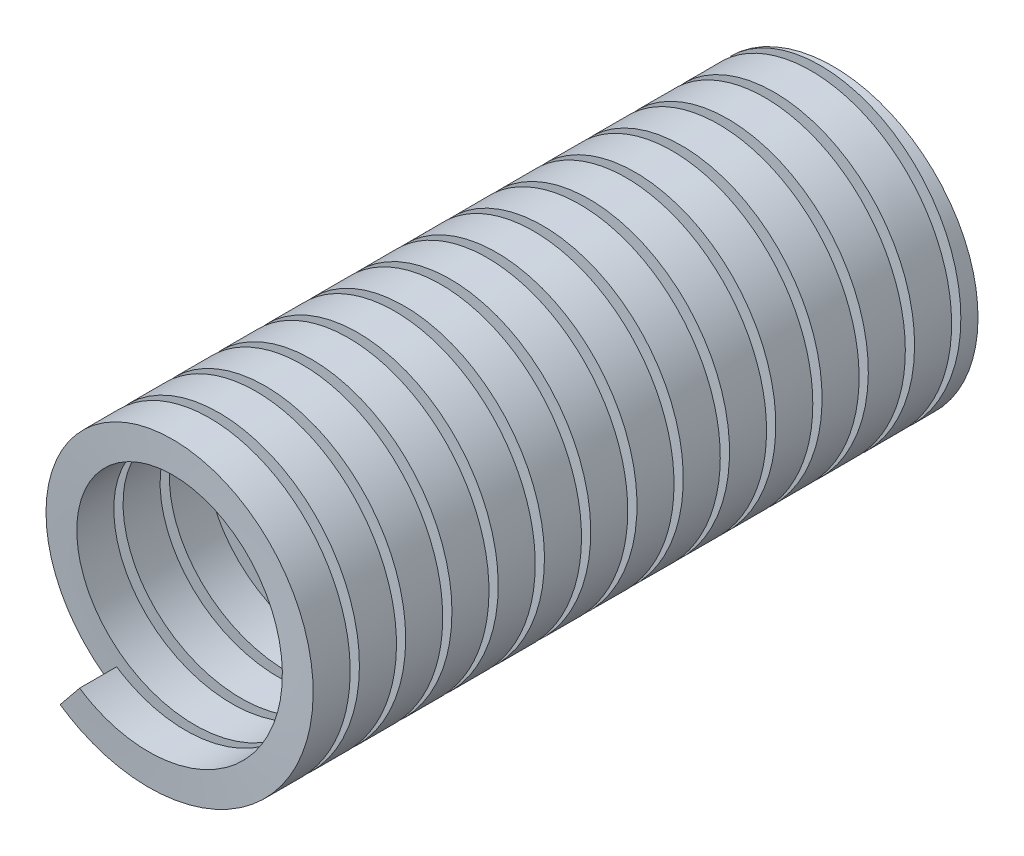
SolidWorks part; units mm, degrees
ref_plane "Front Plane" through (0, 0, 0) normal (0, 0, 1) x (1, 0, 0)
ref_plane "Top Plane" through (0, 0, 0) normal (0, 1, 0) x (1, 0, 0)
ref_plane "Right Plane" through (0, 0, 0) normal (1, 0, 0) x (0, 0, -1)
sketch "Sketch1" plane through (0, 0, 0) normal (0, 0, 1) x (1, 0, 0)
  circle A0 centre (0, 0) radius 47
  dimension "D1" = 94
curve "Helix/Spiral1" pitch 15 height 221 turns 14.7333
sketch "Sketch5" plane through (0, 0, 0) normal (0, 1, 0) x (1, 0, 0)
  line L1 (47, -215.625) -> (37, -215.625)
  line L2 (47, -215.625) -> (47, -203.625)
  line L3 (47, -203.625) -> (37, -203.625)
  line L4 (37, -215.625) -> (37, -203.625)
  line L5 (47, -215.625) -> (37, -203.625) construction
  line L6 (47, -203.625) -> (37, -215.625) construction
  point P0 (42, -209.625)
  dimension "D1" = 10
  dimension "D2" = 12
sweep "Sweep1" add profiles "Sketch5" path "Helix/Spiral1"
sketch "Sketch6" plane through (0, 0, 0) normal (1, 0, 0) x (0, 0, -1)
  line L0 (0, 0) -> (-214.0979, 0) construction
sketch "Sketch7" plane through (0, 0, 0) normal (0, 0, 1) x (1, 0, 0)
  circle A0 centre (0, 0) radius 75
  dimension "D1" = 150
extrude "Cut-Extrude1" cut sketch "Sketch7" against normal blind 60
sketch "Sketch9" plane through (0, 0, 0) normal (0, 0, 1) x (1, 0, 0)
  line L1 (0, 0) -> (0, -33.859) construction
  line L3 (-5, -40.3) -> (5, -40.3)
  line L4 (-5, -40.3) -> (-5, -32.3)
  line L5 (-5, -32.3) -> (5, -32.3)
  line L6 (5, -40.3) -> (5, -32.3)
  dimension "D1" = 10
  dimension "D2" = 8
  dimension "D3" = 40.3
extrude "Cut-Extrude2" cut sketch "Sketch9" along normal blind 55
